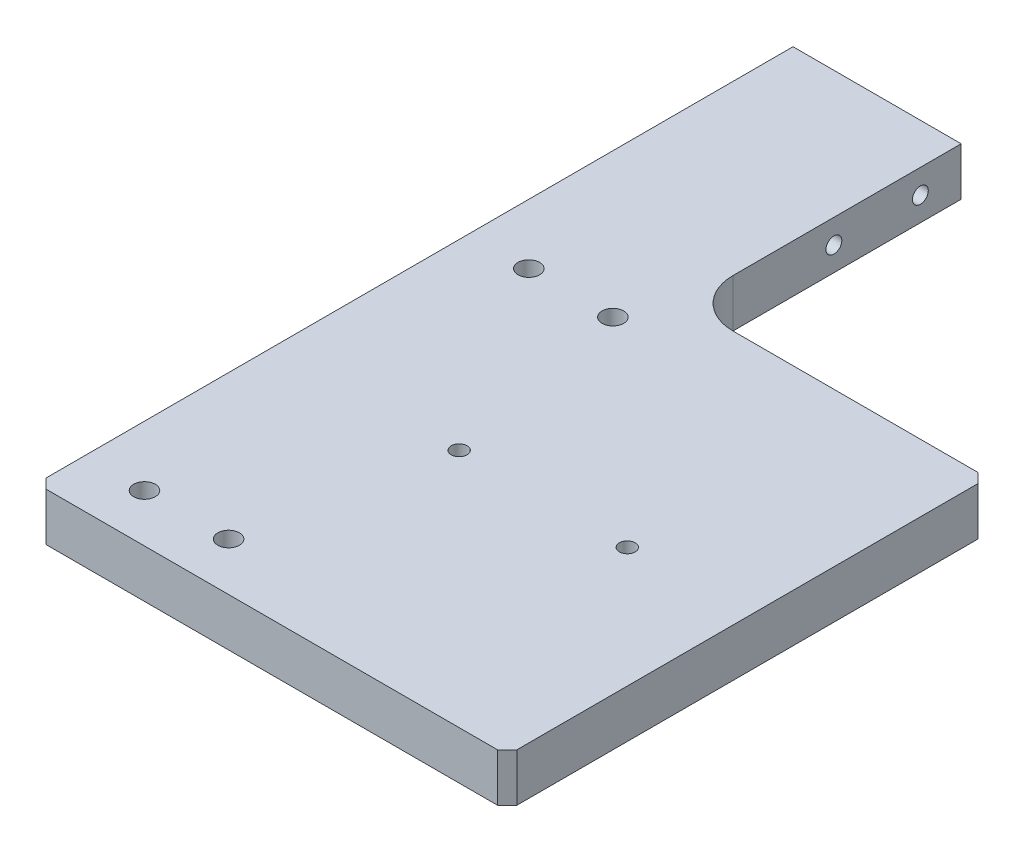
SolidWorks part; units mm, degrees
material "电木（PF）"
ref_plane "前视基准面" through (0, 0, 0) normal (0, 0, 1) x (1, 0, 0)
ref_plane "上视基准面" through (0, 0, 0) normal (0, 1, 0) x (1, 0, 0)
ref_plane "右视基准面" through (0, 0, 0) normal (1, 0, 0) x (0, 0, -1)
sketch "草图2" plane through (0, 0, 0) normal (1, 0, 0) x (0, 0, -1)
  line L1 (-50, 5) -> (50, 5)
  line L2 (-50, 5) -> (-50, -5)
  line L3 (-50, -5) -> (50, -5)
  line L4 (50, 5) -> (50, -5)
  line L5 (-50, 5) -> (50, -5) construction
  line L6 (-50, -5) -> (50, 5) construction
  point P0 (0, 0)
  dimension "D1" = 100
  dimension "D2" = 10
extrude "凸台-拉伸1" add sketch "草图2" along normal blind 98
hole_wizard "M6 螺纹孔1" positions "草图3" profile "草图4" tap size "M6" standard "GB"
sketch "草图3" plane through (0, -5, 0) normal (0, -1, 0) x (-1, 0, 0)
  point P0 (-23, 23.5)
  point P3 (-53, 0)
  point P6 (-23, -23.5)
cosmetic thread "孔螺蚊线1" [suppressed] parameters "D2"=6
cosmetic thread "孔螺蚊线2" [suppressed] parameters "D2"=6
cosmetic thread "孔螺蚊线3" [suppressed] parameters "D2"=6
sketch "草图4" plane through (23, -5, -23.5) normal (1, 0, 0) x (0, 0, -1)
  line L0 (0, 0) -> (0, 10)
  line L1 (0, 10) -> (2.5, 10)
  line L2 (2.5, 10) -> (2.5, 0)
  line L5 (2.5, 0) -> (0, 0)
  line L11 (0, -6.35) -> (0, 107.95) construction
  dimension "通孔螺纹孔钻头直径" = 5
  dimension "通孔螺纹孔钻头深度" = 10
hole_wizard "打孔尺寸(%根据)开槽圆柱头螺钉的类型1" positions "草图5" profile "草图6" counterbore size "M4" standard "GB" end condition through all
sketch "草图5" plane through (0, -5, 0) normal (0, -1, 0) x (-1, 0, 0)
  line L0 (0, -50) -> (0, 50) construction
  line L1 (0, 0) -> (-84.2279, 0) construction
  point P0 (-30, 40)
  point P9 (-30, -40)
  point P11 (-12.5, -40)
  point P12 (-12.5, 40)
  dimension "D1" = 30
  dimension "D2" = 80
  dimension "D3" = 12.5
sketch "草图6" plane through (30, -5, -40) normal (1, 0, 0) x (0, 0, -1)
  line L0 (0, 0) -> (0, 10)
  line L1 (0, 10) -> (2.25, 10)
  line L3 (2.25, 10) -> (2.25, 4.6)
  line L4 (2.25, 4.6) -> (4, 4.6)
  line L5 (4, 4.6) -> (4, 0)
  line L7 (4, 0) -> (0, 0)
  line L11 (0, -6.35) -> (0, 107.95) construction
  dimension "通孔孔直径" = 4.5
  dimension "通孔孔深度" = 10
  dimension "柱形沉头孔直径" = 8
  dimension "柱形沉头孔深度" = 4.6
chamfer "倒角1" distance 2 angle 45 4 edges at (0, 0, -50) (98, 0, -50) (98, 0, 50) (0, 0, 50)
hole_wizard "M4 螺纹孔1" positions "草图7" profile "草图8" tap size "M4" standard "GB" end condition through all
sketch "草图7" plane through (0, -5, 0) normal (0, -1, 0) x (-1, 0, 0)
  point P0 (-73, 0)
  point P2 (-38, 0)
sketch "草图8" plane through (73, -5, 0) normal (1, 0, 0) x (0, 0, -1)
  line L0 (0, 0) -> (0, 10)
  line L1 (0, 10) -> (1.65, 10)
  line L2 (1.65, 10) -> (1.65, 0)
  line L5 (1.65, 0) -> (0, 0)
  line L11 (0, -6.35) -> (0, 107.95) construction
  dimension "通孔螺纹孔钻头直径" = 3.3
  dimension "通孔螺纹孔钻头深度" = 10
cosmetic thread "孔螺蚊线4" parameters "D2"=4
cosmetic thread "孔螺蚊线5" parameters "D2"=4
sketch "草图9" plane through (0, -5, 0) normal (0, -1, 0) x (1, 0, 0)
  line L0 (96, -50) -> (2, -50) construction
  line L1 (0, -48) -> (35, -48)
  line L2 (0, -48) -> (0, -107.5)
  line L3 (0, -107.5) -> (35, -107.5)
  line L4 (35, -48) -> (35, -107.5)
  dimension "D1" = 57.5
  dimension "D2" = 35
extrude "凸台-拉伸2" add sketch "草图9" against normal up to surface (10 mm away) up to face at (73, 5, -1.65)
fillet "圆角1" radius 10 1 edges at (35, 0, -50)
hole_wizard "M4 螺纹孔2" positions "草图10" profile "草图12" tap size "M4" standard "GB"
sketch "草图10" plane through (35, 0, 0) normal (1, 0, 0) x (0, 0, -1)
  point P0 (99, 0)
  point P2 (81, 0)
cosmetic thread "孔螺蚊线6" parameters "D1"=2.4, "D2"=4
cosmetic thread "孔螺蚊线7" parameters "D1"=2.4, "D2"=4
sketch "草图12" plane through (35, 0, -99) normal (0, 1, 0) x (0, 0, -1)
  line L0 (0, 0) -> (0, 12.4914)
  line L1 (0, 12.4914) -> (1.65, 11.5)
  line L2 (1.65, 11.5) -> (1.65, 0)
  line L5 (1.65, 0) -> (0, 0)
  line L10 (0, 12.4914) -> (-1.65, 11.5) construction
  line L11 (0, -6.35) -> (0, 107.95) construction
  dimension "螺纹孔钻头直径" = 3.3
  dimension "螺纹孔钻头深度" = 11.5
  dimension "导头角度" = 118
